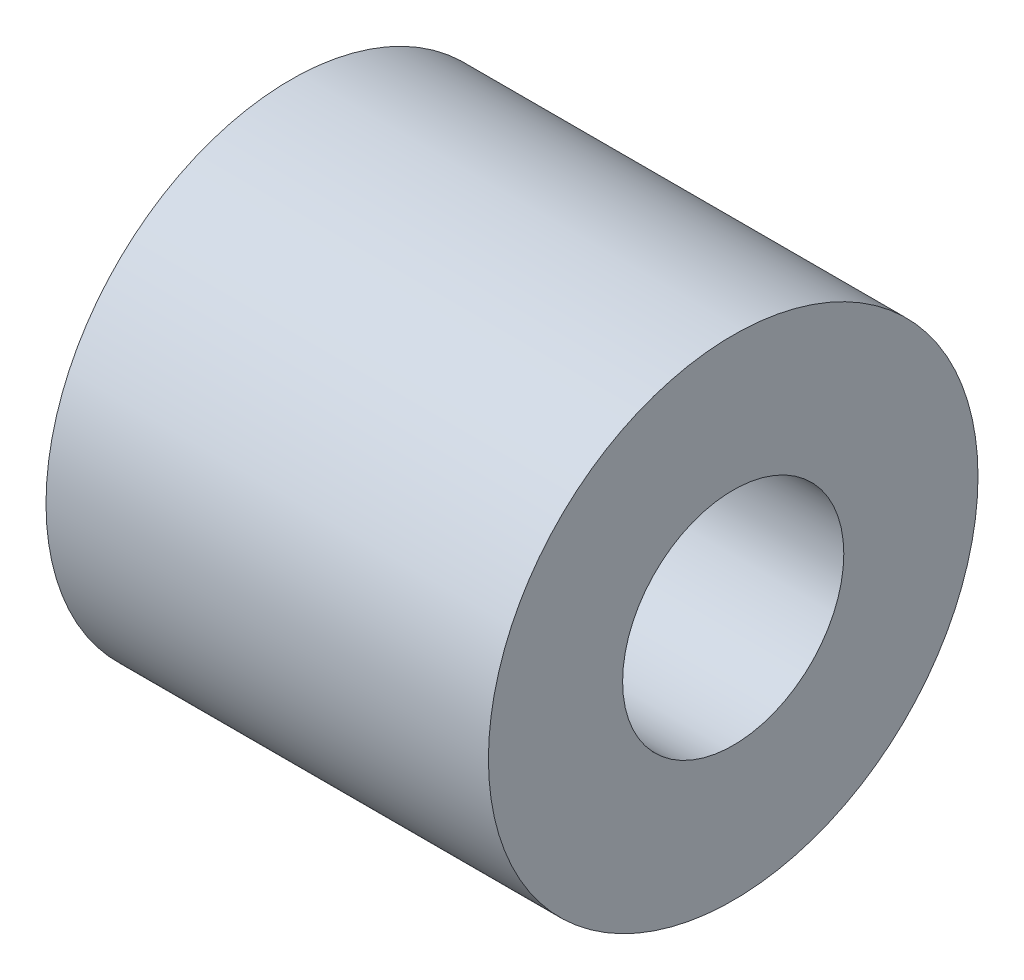
from build123d import *

# Parameters (mm, degrees)
SKETCH1_R           = 830
SKETCH1_R_2         = 375
BOSS_EXTRUDE1_DEPTH = 1500


with BuildPart() as part:
    # Sketch1 → Boss-Extrude1 (new body)
    with BuildSketch(Plane(origin=(0, 0, 0), x_dir=(0, 0, -1), z_dir=(1, 0, 0))):
        Circle(SKETCH1_R)
        Circle(SKETCH1_R_2, mode=Mode.SUBTRACT)
    extrude(amount=BOSS_EXTRUDE1_DEPTH)


solid = part.part
